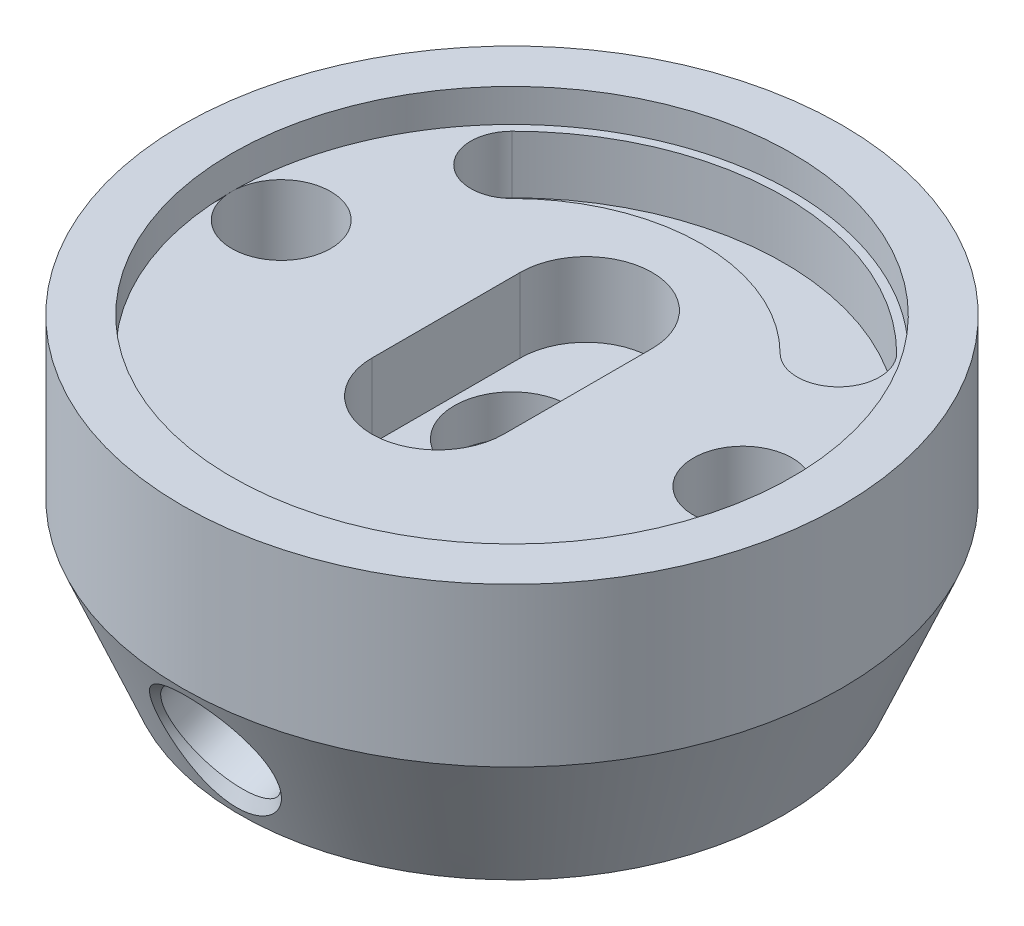
from build123d import *

# Parameters (mm, degrees)
SKETCH2_R                   = 17
CUT_EXTRUDE1_DEPTH          = 2
CUT_EXTRUDE2_DEPTH          = 4.5
CUT_EXTRUDE3_DEPTH          = 3.5
SKETCH5_R                   = 3
CUT_EXTRUDE4_DEPTH          = 11
SKETCH7_R                   = 4.5
CUT_EXTRUDE5_DEPTH          = 6
SKETCH8_R                   = 3.5
CUT_EXTRUDE6_DEPTH          = 2.5
SKETCH9_R                   = 2.6
CUT_EXTRUDE7_DEPTH          = 46.617978912
CHAMFER1_SIZE               = 1
SKETCH10_R                  = 14.5
SKETCH10_R_2                = 6.5
CUT_EXTRUDE8_DEPTH          = 0.5
M8_TAPPED_HOLE1_D           = 6.8
M8_TAPPED_HOLE1_DEPTH       = 10
M8_TAPPED_HOLE1_CSINK_D     = 8.05
M8_TAPPED_HOLE1_CSINK_ANGLE = 90
M8_TAPPED_HOLE1_TIP         = 2.042926105


with BuildPart() as part:
    # Sketch1 → Revolve1 (revolve)
    with BuildSketch(Plane.XY, mode=Mode.PRIVATE) as revolve1_sk:
        Polygon((0, 9.6), (0, 0), (3.5, -8.4), (20, -8.4), (20, 9.6), align=None)
    revolve(revolve1_sk.sketch.rotate(Axis((20, -8.4, 0), (0, 1, 0)), 180), axis=Axis((20, -8.4, 0), (0, 1, 0)))

    # Sketch2 → Cut-Extrude1 (cut)
    with BuildSketch(Plane(origin=(0, 9.6, 0), x_dir=(1, 0, 0), z_dir=(0, 1, 0))):
        with Locations(Location((20, 0, 0), (0, 0, 180))):
            Circle(SKETCH2_R)
    extrude(amount=-CUT_EXTRUDE1_DEPTH, mode=Mode.SUBTRACT)

    # Sketch3 → Cut-Extrude2 (cut)
    with BuildSketch(Plane(origin=(0, 7.6, 0), x_dir=(1, 0, 0), z_dir=(0, 1, 0))):
        with BuildLine():
            Line((24, 4.5), (24, -4.5))
            ThreePointArc((24, -4.5), (20, -8.5), (16, -4.5))
            Line((16, -4.5), (16, 4.5))
            ThreePointArc((16, 4.5), (20, 8.5), (24, 4.5))
        make_face()
    extrude(amount=-CUT_EXTRUDE2_DEPTH, mode=Mode.SUBTRACT)

    # Sketch4 → Cut-Extrude3 (cut)
    with BuildSketch(Plane(origin=(0, 7.6, 0), x_dir=(1, 0, 0), z_dir=(0, 1, 0))):
        with BuildLine():
            ThreePointArc((31.66726189, 11.66726189), (20, 16.5), (8.33273811, 11.66726189))
            ThreePointArc((8.33273811, 11.66726189), (8.33273811, 8.131727984), (11.868272016, 8.131727984))
            ThreePointArc((11.868272016, 8.131727984), (20, 11.5), (28.131727984, 8.131727984))
            ThreePointArc((28.131727984, 8.131727984), (31.66726189, 8.131727984), (31.66726189, 11.66726189))
        make_face()
    extrude(amount=-CUT_EXTRUDE3_DEPTH, mode=Mode.SUBTRACT)

    # Sketch5 → Cut-Extrude4 (cut)
    with BuildSketch(Plane(origin=(0, 7.6, 0), x_dir=(1, 0, 0), z_dir=(0, 1, 0))):
        with Locations(Location((6, 0, 0), (0, 0, 180))):
            Circle(SKETCH5_R)
        with Locations((34, 0)):
            Circle(SKETCH5_R)
    extrude(amount=-CUT_EXTRUDE4_DEPTH, mode=Mode.SUBTRACT)

    # Sketch7 → Cut-Extrude5 (cut)
    with BuildSketch(Plane.XZ.offset(8.4)):
        with Locations((20, 0)):
            Circle(SKETCH7_R)
    extrude(amount=-CUT_EXTRUDE5_DEPTH, mode=Mode.SUBTRACT)

    # Sketch8 → Cut-Extrude6 (cut)
    with BuildSketch(Plane(origin=(0, 3.1, 0), x_dir=(1, 0, 0), z_dir=(0, 1, 0))):
        with Locations(Location((20, 0, 0), (0, 0, 180))):
            Circle(SKETCH8_R)
    extrude(amount=-CUT_EXTRUDE6_DEPTH, mode=Mode.SUBTRACT)

    # Sketch9 → Cut-Extrude7 (cut, through all)
    with BuildSketch(Plane(origin=(0, 0.6, 0), x_dir=(1, 0, 0), z_dir=(0, 1, 0))):
        with Locations(Location((20, 0, 0), (0, 0, 180))):
            Circle(SKETCH9_R)
    extrude(amount=-CUT_EXTRUDE7_DEPTH, mode=Mode.SUBTRACT)

    # Chamfer1
    chamfer1_edges = [part.edges().sort_by_distance(p)[0] for p in [
        (22.6, -2.4, 0),
    ]]
    chamfer(chamfer1_edges, length=CHAMFER1_SIZE)

    # Sketch10 → Cut-Extrude8 (cut)
    with BuildSketch(Plane.XZ.offset(8.4)):
        with Locations((20, 0)):
            Circle(SKETCH10_R)
        with Locations((20, 0)):
            Circle(SKETCH10_R_2, mode=Mode.SUBTRACT)
    extrude(amount=-CUT_EXTRUDE8_DEPTH, mode=Mode.SUBTRACT)

    # M8 Tapped Hole1
    with Locations(Plane(origin=(0, -7.100591716, 17.041420118), x_dir=(1, 0, 0), z_dir=(0, -0.38461538461538547, 0.9230769230769227))):
        with Locations((20, 3.142307692)):
            CounterSinkHole(M8_TAPPED_HOLE1_D / 2, M8_TAPPED_HOLE1_CSINK_D / 2, depth=M8_TAPPED_HOLE1_DEPTH, counter_sink_angle=M8_TAPPED_HOLE1_CSINK_ANGLE)
            with Locations((0, 0, -(M8_TAPPED_HOLE1_DEPTH + M8_TAPPED_HOLE1_TIP / 2))):  # 118° drill point
                Cone(0, M8_TAPPED_HOLE1_D / 2, M8_TAPPED_HOLE1_TIP, mode=Mode.SUBTRACT)


solid = part.part
